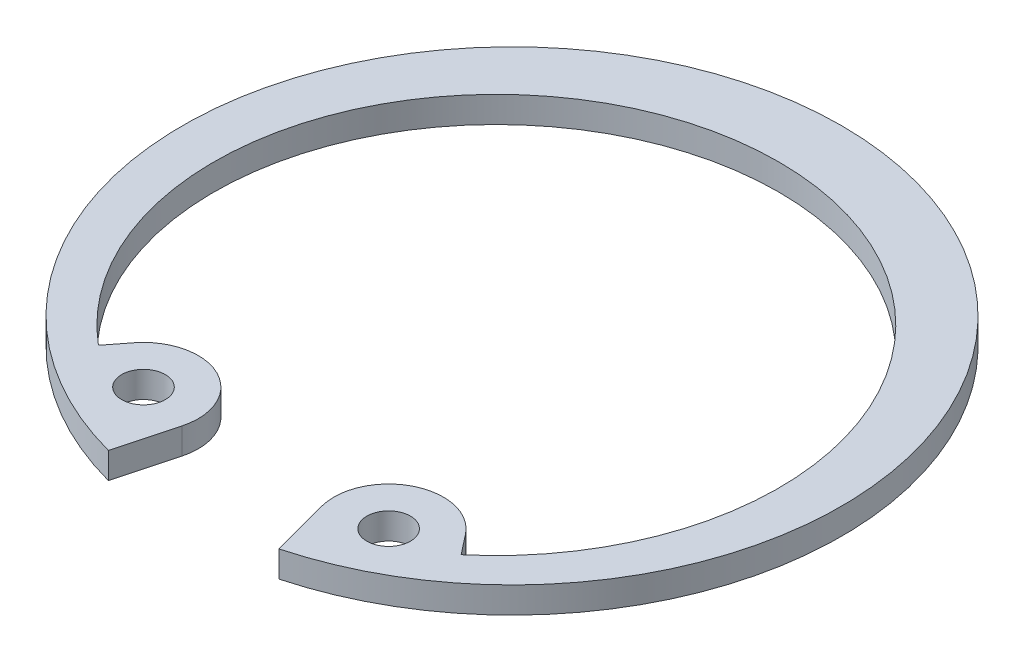
from build123d import *

# Parameters (mm, degrees)
SKETCH2_R           = 1.25
BOSS_EXTRUDE1_DEPTH = 1.5


with BuildPart() as part:
    # Sketch2 → Boss-Extrude1 (new body)
    with BuildSketch(Plane(origin=(0, 0, 0), x_dir=(1, 0, 0), z_dir=(0, 1, 0))):
        with BuildLine():
            Line((-10.401091034, -13.320036445), (-9.505079721, -12.172569963))
            ThreePointArc((-9.505079721, -12.172569963), (-5.62952549, -11.294814862), (-3.997208572, -14.91778548))
            Line((-3.997208572, -14.91778548), (-4.891679952, -18.255998117))
            ThreePointArc((-4.891679952, -18.255998117), (0, 18.9), (4.891679952, -18.255998117))
            Line((4.891679952, -18.255998117), (3.997208572, -14.91778548))
            ThreePointArc((3.997208572, -14.91778548), (5.62952549, -11.294814862), (9.505079721, -12.172569963))
            Line((9.505079721, -12.172569963), (10.401091034, -13.320036445))
            ThreePointArc((10.401091034, -13.320036445), (0, 15.3), (-10.401091034, -13.320036445))
        make_face()
        with Locations(Location((-7.030215667, -14.105093678, 0), (0, 0, 270))):
            Circle(SKETCH2_R, mode=Mode.SUBTRACT)
        with Locations(Location((7.030215667, -14.105093678, 0), (0, 0, 90))):
            Circle(SKETCH2_R, mode=Mode.SUBTRACT)
    extrude(amount=BOSS_EXTRUDE1_DEPTH)


solid = part.part
